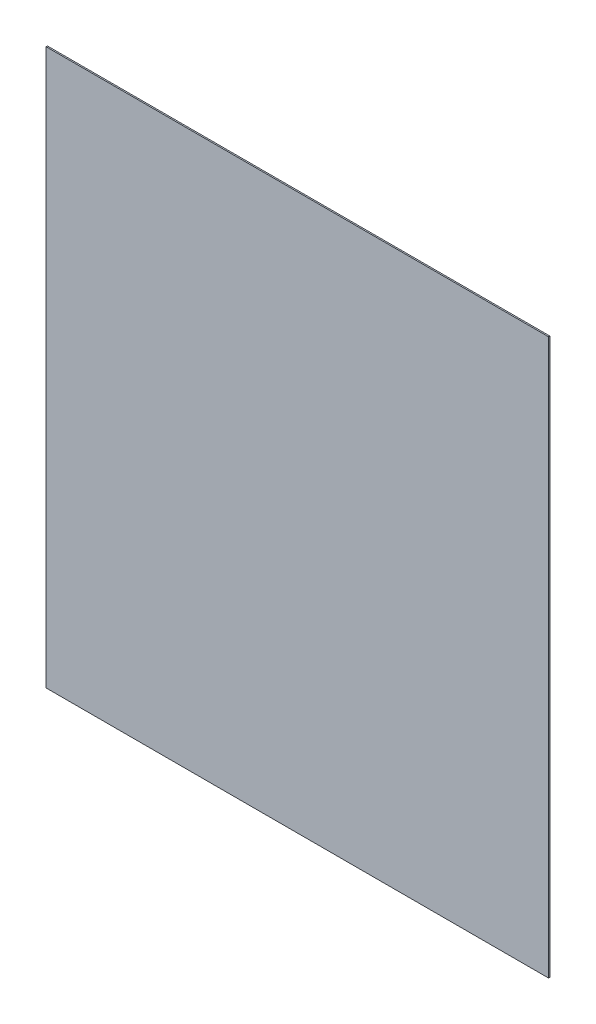
from build123d import *

# Parameters (mm, degrees)
SKETCH_1_W      = 1135
SKETCH_1_H      = 1255
EXTRUDE_1_DEPTH = 3


with BuildPart() as part:
    # 草图1 → 凸台-拉伸1 (new body)
    with BuildSketch(Plane.XY):
        Rectangle(SKETCH_1_W, SKETCH_1_H)
    extrude(amount=EXTRUDE_1_DEPTH)


solid = part.part
